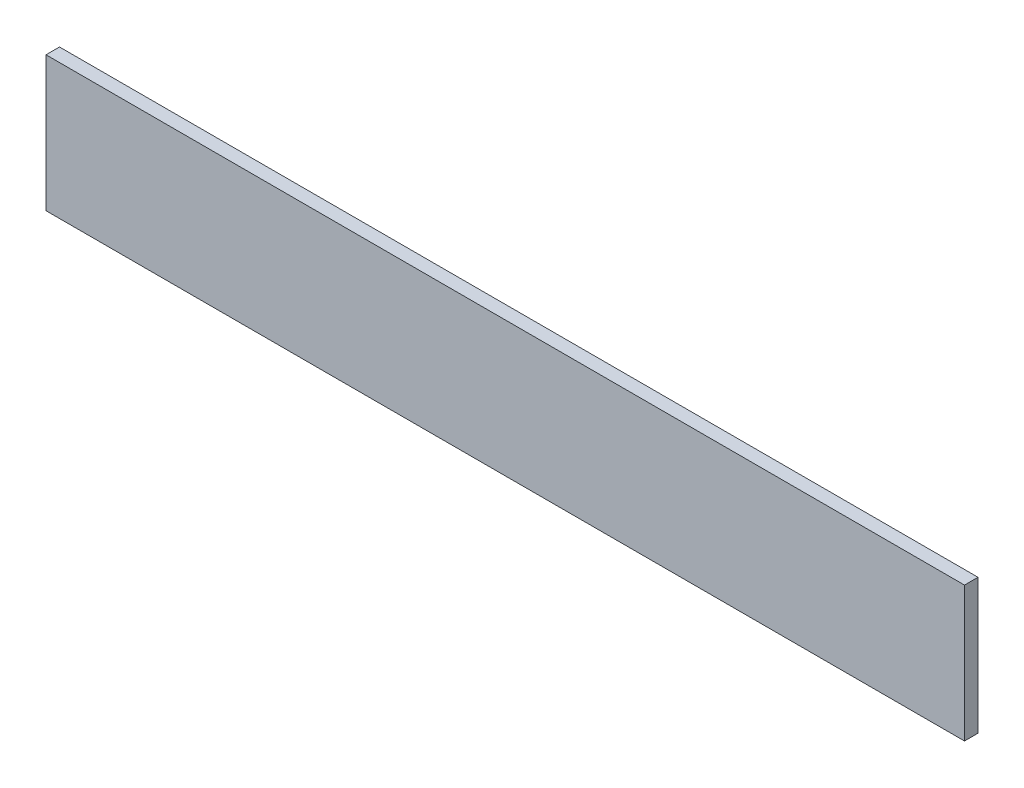
SolidWorks part; units mm, degrees
ref_plane "前视基准面" through (0, 0, 0) normal (0, 0, 1) x (1, 0, 0)
ref_plane "上视基准面" through (0, 0, 0) normal (0, 1, 0) x (1, 0, 0)
ref_plane "右视基准面" through (0, 0, 0) normal (1, 0, 0) x (0, 0, -1)
sketch "草图1" plane through (0, 0, 0) normal (0, 0, 1) x (1, 0, 0)
  line L0 (0, 0) -> (340, 0)
  line L1 (340, 0) -> (340, 50)
  line L2 (340, 50) -> (0, 50)
  line L3 (0, 50) -> (0, 0)
extrude "凸台-拉伸1" add sketch "草图1" along normal blind 5
